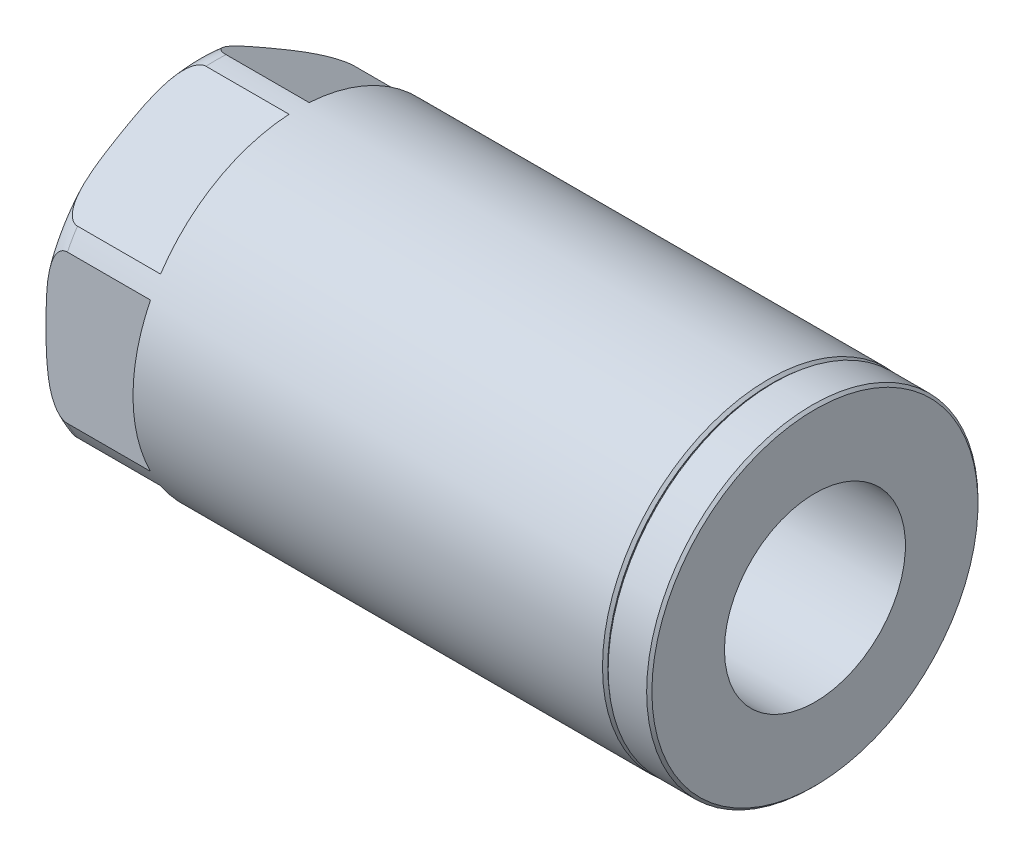
from build123d import *

# Parameters (mm, degrees)
SKETCH2_W          = 68
SKETCH2_H          = 68
CUT_EXTRUDE1_DEPTH = 12


with BuildPart() as part:
    # Sketch1 → Revolve1 (revolve)
    with BuildSketch(Plane.XY, mode=Mode.PRIVATE) as revolve1_sk:
        with BuildLine():
            Line((0, 0), (0, 16.5))
            ThreePointArc((0, 16.5), (0.732233047, 18.267766953), (2.5, 19))
            Line((2.5, 19), (65.7, 19))
            Line((65.7, 19), (66, 18.7))
            Line((66, 18.7), (66, 18.65))
            Line((66, 18.65), (66.3, 18.95))
            Line((66.3, 18.95), (70.7, 18.95))
            Line((70.7, 18.95), (71, 18.65))
            Line((71, 18.65), (71, 0))
            Line((71, 0), (0, 0))
        make_face()
    revolve(revolve1_sk.sketch.rotate(Axis((71, 0, 0), (-1, 0, 0)), 270), axis=Axis((71, 0, 0), (-1, 0, 0)))

    # Sketch2 → Cut-Extrude1 (cut)
    with BuildSketch(Plane(origin=(0, 0, 0), x_dir=(0, 0, -1), z_dir=(1, 0, 0))):
        Rectangle(SKETCH2_W, SKETCH2_H)
        Polygon((-17, -9.814954576), (0, -19.629909152), (17, -9.814954576), (17, 9.814954576), (0, 19.629909152), (-17, 9.814954576), align=None, mode=Mode.SUBTRACT)
    extrude(amount=CUT_EXTRUDE1_DEPTH, mode=Mode.SUBTRACT)

    # Sketch3 → Cut-Revolve1 (revolve, cut)
    with BuildSketch(Plane.XY, mode=Mode.PRIVATE) as cut_revolve1_sk:
        Polygon((0, 0), (0, 8), (0.812, 7.188), (8.174418449, 7.188), (10, 10.35), (71, 10.35), (71, 0), align=None)
    revolve(cut_revolve1_sk.sketch.rotate(Axis((71, 0, 0), (-1, 0, 0)), 270), axis=Axis((71, 0, 0), (-1, 0, 0)), mode=Mode.SUBTRACT)


solid = part.part
